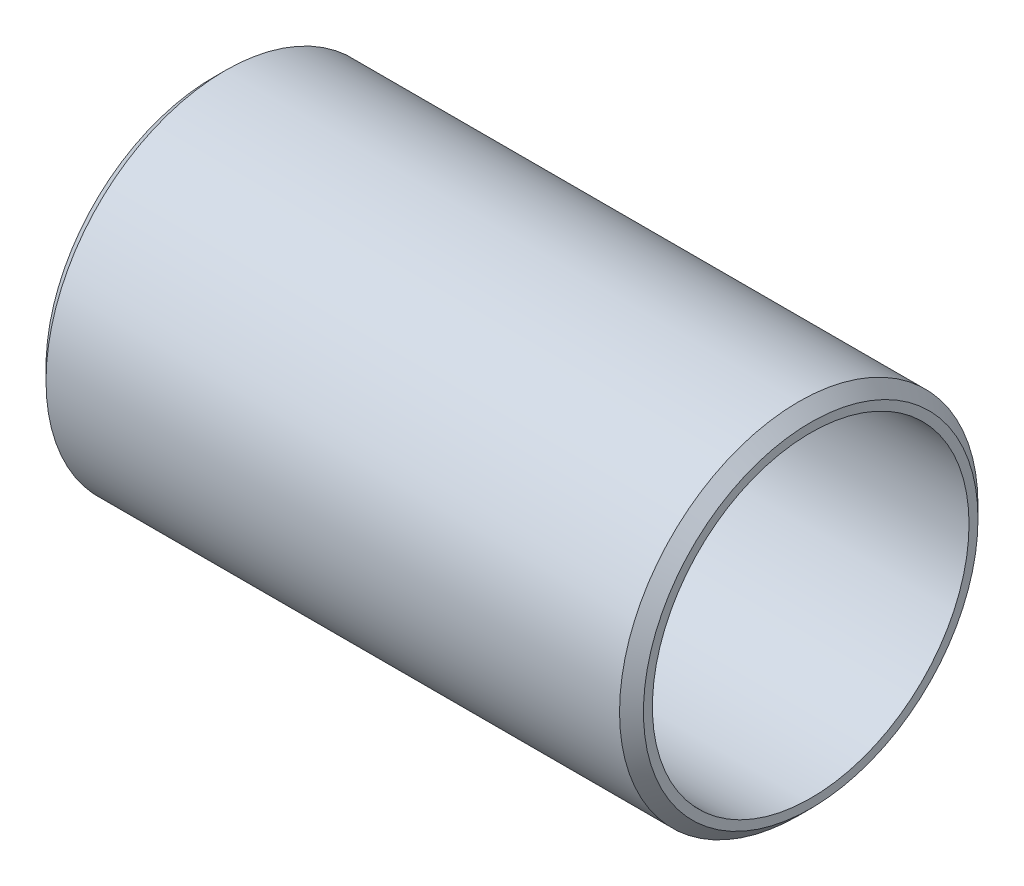
SolidWorks part; units mm, degrees
material "镀锌焊接钢管 Q215A"
ref_plane "前视基准面" through (0, 0, 0) normal (0, 0, 1) x (1, 0, 0)
ref_plane "上视基准面" through (0, 0, 0) normal (0, 1, 0) x (1, 0, 0)
ref_plane "右视基准面" through (0, 0, 0) normal (1, 0, 0) x (0, 0, -1)
sketch "草图1" plane through (0, 0, 0) normal (1, 0, 0) x (0, 0, -1)
  circle A0 centre (0, 0) radius 30
  dimension "D1" = 60
extrude "拉伸-薄壁1" add sketch "草图1" along normal blind 100 thin thin type one direction reverse wall 3.5
cosmetic thread "装饰螺纹线1" parameters "D1"=30, "D2"=56.656
cosmetic thread "装饰螺纹线2" parameters "D1"=30, "D2"=56.656
chamfer "倒角1" distance 2 angle 45 2 edges at (100, 0, -30) (0, 0, -30)
